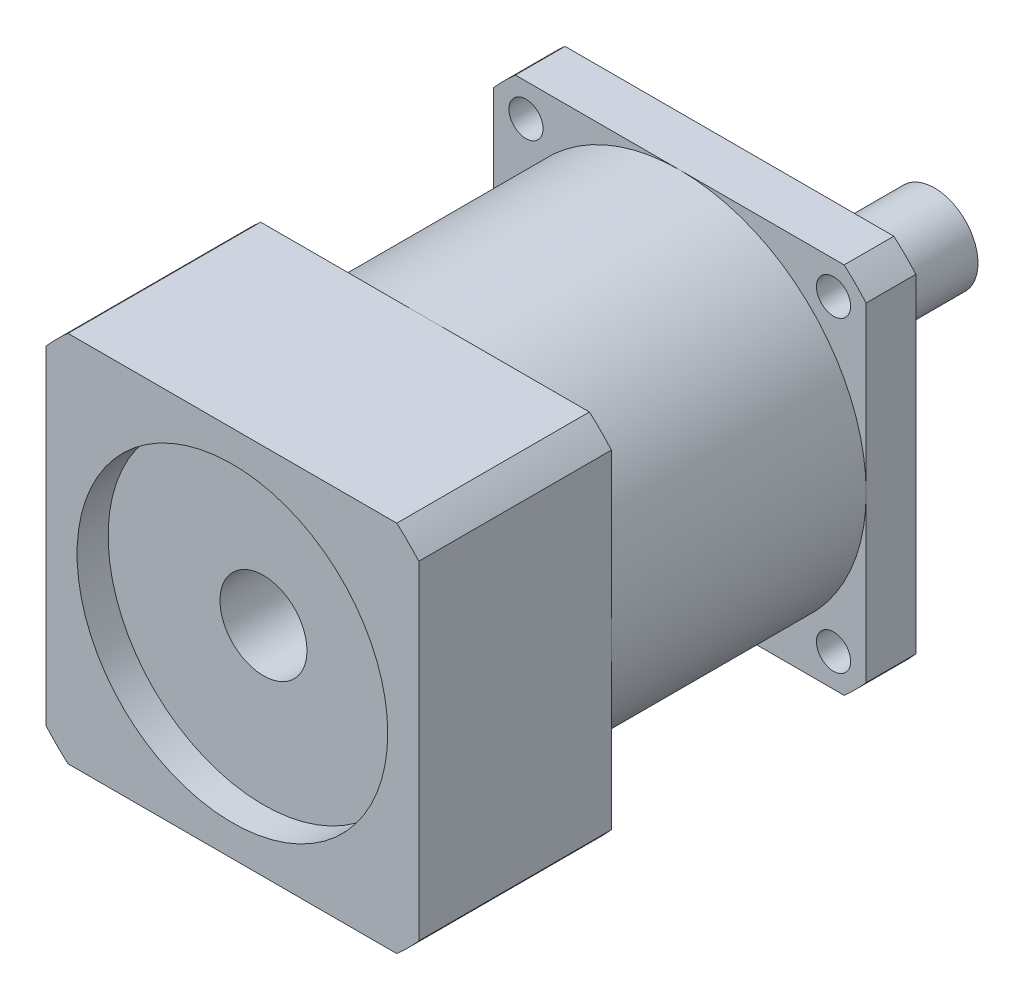
from build123d import *

# Parameters (mm, degrees)
SKETCH_1_R          = 7
EXTRUDE_1_DEPTH     = 30
SKETCH_2_R          = 25
EXTRUDE_2_DEPTH     = 3
SKETCH_3_W          = 60
SKETCH_3_H          = 60
EXTRUDE_3_DEPTH     = 8
SKETCH_4_R          = 30
EXTRUDE_4_DEPTH     = 41
SKETCH_5_W          = 60
SKETCH_5_H          = 60
EXTRUDE_5_DEPTH     = 31
SKETCH_6_W          = 7.340334956
SKETCH_6_H          = 80
CUT_EXTRUDE_1_REACH = 92.554
SKETCH_7_R          = 2.75
CUT_EXTRUDE_START   = -5
SKETCH_8_R          = 25
CUT_EXTRUDE_2_DEPTH = 5
CUT_EXTRUDE_START_2 = -25
SKETCH_9_R          = 7
CUT_EXTRUDE_3_DEPTH = 25


with BuildPart() as part:
    # 草图1 → 凸台-拉伸1 (new body)
    with BuildSketch(Plane.XY):
        Circle(SKETCH_1_R)
    extrude(amount=EXTRUDE_1_DEPTH)

    # 草图2 → 凸台-拉伸2 (add)
    with BuildSketch(Plane.XY.offset(30)):
        Circle(SKETCH_2_R)
    extrude(amount=EXTRUDE_2_DEPTH)

    # 草图3 → 凸台-拉伸3 (add)
    with BuildSketch(Plane.XY.offset(33)):
        Rectangle(SKETCH_3_W, SKETCH_3_H)
    extrude(amount=EXTRUDE_3_DEPTH)

    # 草图4 → 凸台-拉伸4 (add)
    with BuildSketch(Plane.XY.offset(41)):
        Circle(SKETCH_4_R)
    extrude(amount=EXTRUDE_4_DEPTH)

    # 草图5 → 凸台-拉伸5 (add)
    with BuildSketch(Plane.XY.offset(82)):
        Rectangle(SKETCH_5_W, SKETCH_5_H)
    extrude(amount=EXTRUDE_5_DEPTH)

    # 草图6 → 切除-旋转1 (revolve, cut)
    with BuildSketch(Plane(origin=(0, 0, 0), x_dir=(1, 0, 0), z_dir=(0, 1, 0))):
        with Locations((-43.670167478, -73)):
            Rectangle(SKETCH_6_W, SKETCH_6_H)
    revolve(axis=Axis((0, 0, 82), (0, 0, -1)), mode=Mode.SUBTRACT)

    # 草图7 → 切除-拉伸1 (cut, up to next)
    with BuildSketch(Plane(origin=(0, 0, 33), x_dir=(-1, 0, 0), z_dir=(0, 0, -1)), mode=Mode.PRIVATE) as cut_extrude_1_sk1:
        with Locations((-24.748737342, 24.748737342)):
            Circle(SKETCH_7_R)
    cut_extrude_1_tool1 = extrude(cut_extrude_1_sk1.sketch, amount=-CUT_EXTRUDE_1_REACH, mode=Mode.PRIVATE) & part.part
    # 草图7 → 切除-拉伸1 (cut, up to next)
    with BuildSketch(Plane(origin=(0, 0, 33), x_dir=(-1, 0, 0), z_dir=(0, 0, -1)), mode=Mode.PRIVATE) as cut_extrude_1_sk2:
        with Locations(Location((24.748737342, 24.748737342, 0), (0, 0, 180))):
            Circle(SKETCH_7_R)
    cut_extrude_1_tool2 = extrude(cut_extrude_1_sk2.sketch, amount=-CUT_EXTRUDE_1_REACH, mode=Mode.PRIVATE) & part.part
    # 草图7 → 切除-拉伸1 (cut, up to next)
    with BuildSketch(Plane(origin=(0, 0, 33), x_dir=(-1, 0, 0), z_dir=(0, 0, -1)), mode=Mode.PRIVATE) as cut_extrude_1_sk3:
        with Locations(Location((-24.748737342, -24.748737342, 0), (0, 0, 180))):
            Circle(SKETCH_7_R)
    cut_extrude_1_tool3 = extrude(cut_extrude_1_sk3.sketch, amount=-CUT_EXTRUDE_1_REACH, mode=Mode.PRIVATE) & part.part
    # 草图7 → 切除-拉伸1 (cut, up to next)
    with BuildSketch(Plane(origin=(0, 0, 33), x_dir=(-1, 0, 0), z_dir=(0, 0, -1)), mode=Mode.PRIVATE) as cut_extrude_1_sk4:
        with Locations((24.748737342, -24.748737342)):
            Circle(SKETCH_7_R)
    cut_extrude_1_tool4 = extrude(cut_extrude_1_sk4.sketch, amount=-CUT_EXTRUDE_1_REACH, mode=Mode.PRIVATE) & part.part
    add(cut_extrude_1_tool1.solids().sort_by_distance((24.748737, 24.748737, 33))[0], mode=Mode.SUBTRACT)
    add(cut_extrude_1_tool2.solids().sort_by_distance((-24.748737, 24.748737, 33))[0], mode=Mode.SUBTRACT)
    add(cut_extrude_1_tool3.solids().sort_by_distance((24.748737, -24.748737, 33))[0], mode=Mode.SUBTRACT)
    add(cut_extrude_1_tool4.solids().sort_by_distance((-24.748737, -24.748737, 33))[0], mode=Mode.SUBTRACT)

    # 草图8 → 切除-拉伸2 (cut)
    with BuildSketch(Plane.XY.offset(113).offset(CUT_EXTRUDE_START)):
        Circle(SKETCH_8_R)
    extrude(amount=CUT_EXTRUDE_2_DEPTH, mode=Mode.SUBTRACT)

    # 草图9 → 切除-拉伸3 (cut)
    with BuildSketch(Plane.XY.offset(108).offset(CUT_EXTRUDE_START_2)):
        Circle(SKETCH_9_R)
    extrude(amount=CUT_EXTRUDE_3_DEPTH, mode=Mode.SUBTRACT)


solid = part.part
